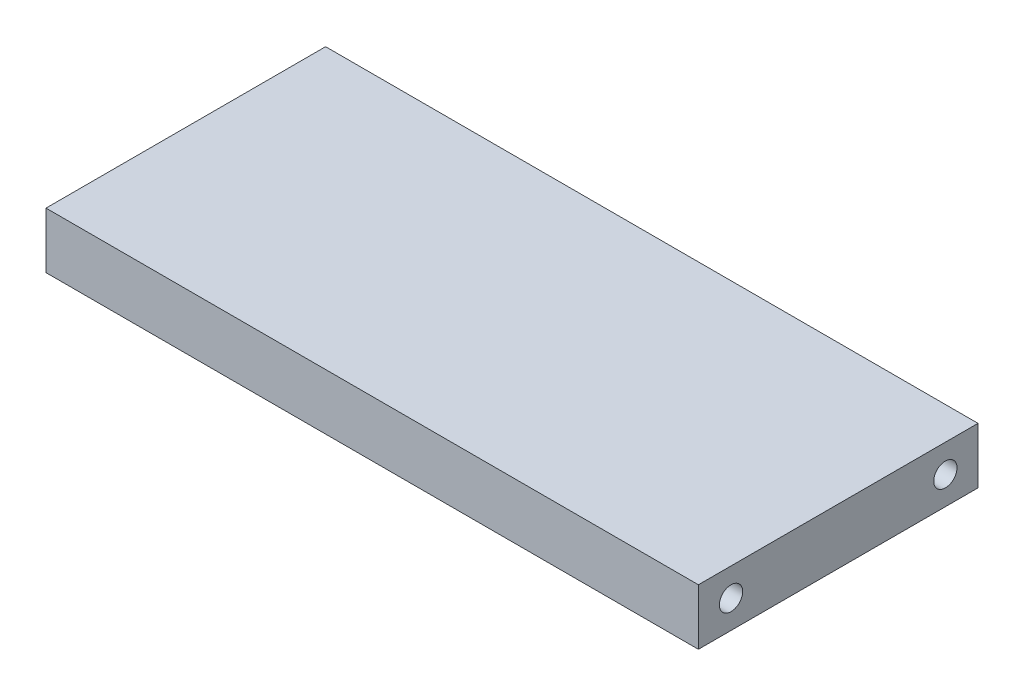
SolidWorks part; units mm, degrees
material "Q235B"
ref_plane "Front Plane" through (0, 0, 0) normal (0, 0, 1) x (1, 0, 0)
ref_plane "Top Plane" through (0, 0, 0) normal (0, 1, 0) x (1, 0, 0)
ref_plane "Right Plane" through (0, 0, 0) normal (1, 0, 0) x (0, 0, -1)
sketch "Sketch1" plane through (0, 0, 0) normal (0, 1, 0) x (1, 0, 0)
  line L1 (-35, 15) -> (35, 15)
  line L2 (-35, 15) -> (-35, -15)
  line L3 (-35, -15) -> (35, -15)
  line L4 (35, 15) -> (35, -15)
  line L5 (-35, 15) -> (35, -15) construction
  line L6 (-35, -15) -> (35, 15) construction
  point P0 (0, 0)
  dimension "D1" = 30
  dimension "D2" = 70
extrude "Boss-Extrude1" add sketch "Sketch1" along normal blind 6
sketch "Sketch2" plane through (35, 0, 0) normal (1, 0, 0) x (0, 0, -1)
  circle A0 centre (11.5, 3) radius 1.25
  circle A1 centre (-11.5, 3) radius 1.25
  dimension "D1" = 2.5
extrude "Cut-Extrude1" cut sketch "Sketch2" against normal blind 5
sketch "Sketch3" plane through (-35, 0, 0) normal (-1, 0, 0) x (0, 0, 1)
  circle A0 centre (-11.5, 3) radius 1.25
  circle A1 centre (11.5, 3) radius 1.25
  dimension "D1" = 2.5
extrude "Cut-Extrude2" cut sketch "Sketch3" against normal blind 5
